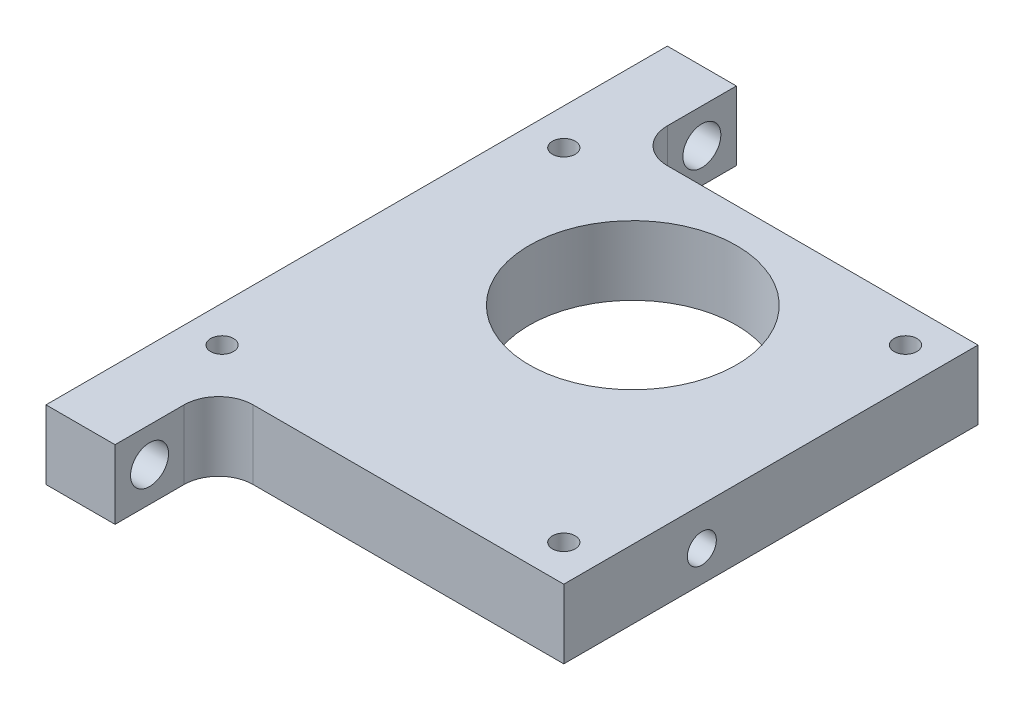
from build123d import *

# Parameters (mm, degrees)
SKETCH1_W                      = 60
SKETCH1_H                      = 90
BOSS_EXTRUDE1_DEPTH            = 10
SKETCH4_R                      = 15
CUT_EXTRUDE3_DEPTH             = 56
M4_TAPPED_HOLE1_D              = 3.3
SKETCH8_W                      = 50
SKETCH8_H                      = 15
CUT_EXTRUDE5_DEPTH             = 56
F_5_5_5_5_DIAMETER_HOLE1_D     = 5.5
F_5_5_5_5_DIAMETER_HOLE1_DEPTH = 12.4
F_5_5_5_5_DIAMETER_HOLE1_TIP   = 1.652366702
FILLET1_R                      = 5
M5_TAPPED_HOLE1_D              = 4.2
M5_TAPPED_HOLE1_DEPTH          = 12.4
M5_TAPPED_HOLE1_TIP            = 1.2618073


with BuildPart() as part:
    # Sketch1 → Boss-Extrude1 (new body)
    with BuildSketch(Plane(origin=(0, 0, 0), x_dir=(1, 0, 0), z_dir=(0, 1, 0))):
        Rectangle(SKETCH1_W, SKETCH1_H)
    extrude(amount=BOSS_EXTRUDE1_DEPTH)

    # Sketch4 → Cut-Extrude3 (cut, through all)
    with BuildSketch(Plane.XZ):
        with Locations(Location((0, -10, 0), (0, 0, 270))):
            Circle(SKETCH4_R)
    extrude(amount=-CUT_EXTRUDE3_DEPTH, mode=Mode.SUBTRACT)

    # M4 Tapped Hole1 (through all)
    with Locations(Plane.XZ):
        with Locations((-24.748737342, 24.747474683), (-24.748737342, -24.75), (24.748737342, -24.75), (24.748737342, 24.747474683)):
            Hole(M4_TAPPED_HOLE1_D / 2)

    # Sketch8 → Cut-Extrude5 (cut, through all)
    with BuildSketch(Plane.XZ):
        with Locations((5, 37.5)):
            Rectangle(SKETCH8_W, SKETCH8_H)
        with Locations((5, -37.5)):
            Rectangle(SKETCH8_W, SKETCH8_H)
    extrude(amount=-CUT_EXTRUDE5_DEPTH, mode=Mode.SUBTRACT)

    # Ø5.5 (5.5) Diameter Hole1
    with Locations(Plane.ZY.offset(30)):
        with Locations((-40, 5), (40, 5)):
            Hole(F_5_5_5_5_DIAMETER_HOLE1_D / 2, depth=F_5_5_5_5_DIAMETER_HOLE1_DEPTH)
            with Locations((0, 0, -(F_5_5_5_5_DIAMETER_HOLE1_DEPTH + F_5_5_5_5_DIAMETER_HOLE1_TIP / 2))):  # 118° drill point
                Cone(0, F_5_5_5_5_DIAMETER_HOLE1_D / 2, F_5_5_5_5_DIAMETER_HOLE1_TIP, mode=Mode.SUBTRACT)

    # Fillet1
    fillet1_edges = [part.edges().sort_by_distance(p)[0] for p in [
        (-20, 5, 30),
        (-20, 5, -30),
    ]]
    fillet(fillet1_edges, radius=FILLET1_R)

    # M5 Tapped Hole1
    with Locations(Plane(origin=(30, 0, 0), x_dir=(0, 0, -1), z_dir=(1, 0, 0))):
        with Locations((-10.000955133, 4.5)):
            Hole(M5_TAPPED_HOLE1_D / 2, depth=M5_TAPPED_HOLE1_DEPTH)
            with Locations((0, 0, -(M5_TAPPED_HOLE1_DEPTH + M5_TAPPED_HOLE1_TIP / 2))):  # 118° drill point
                Cone(0, M5_TAPPED_HOLE1_D / 2, M5_TAPPED_HOLE1_TIP, mode=Mode.SUBTRACT)


solid = part.part
